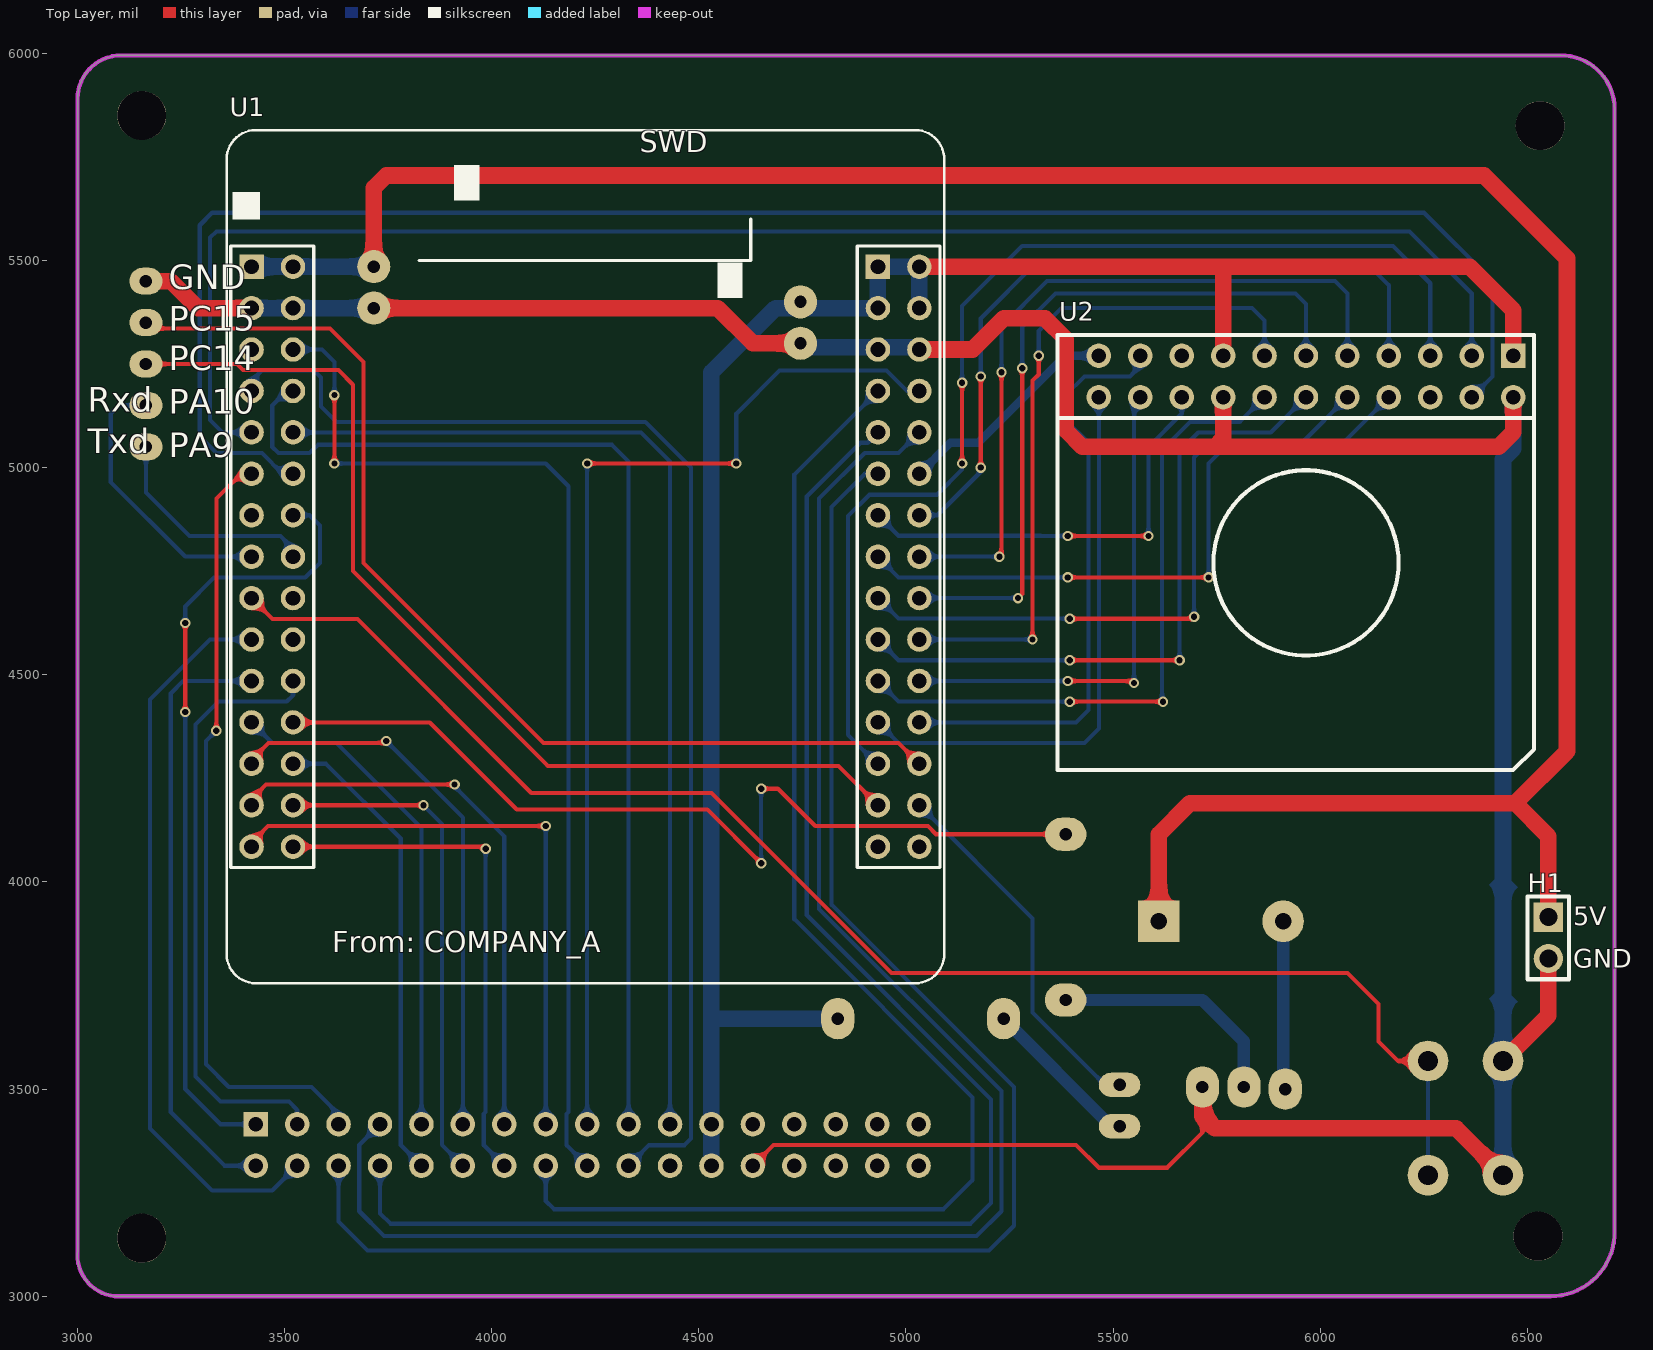
[diagram p0: Top Layer view]
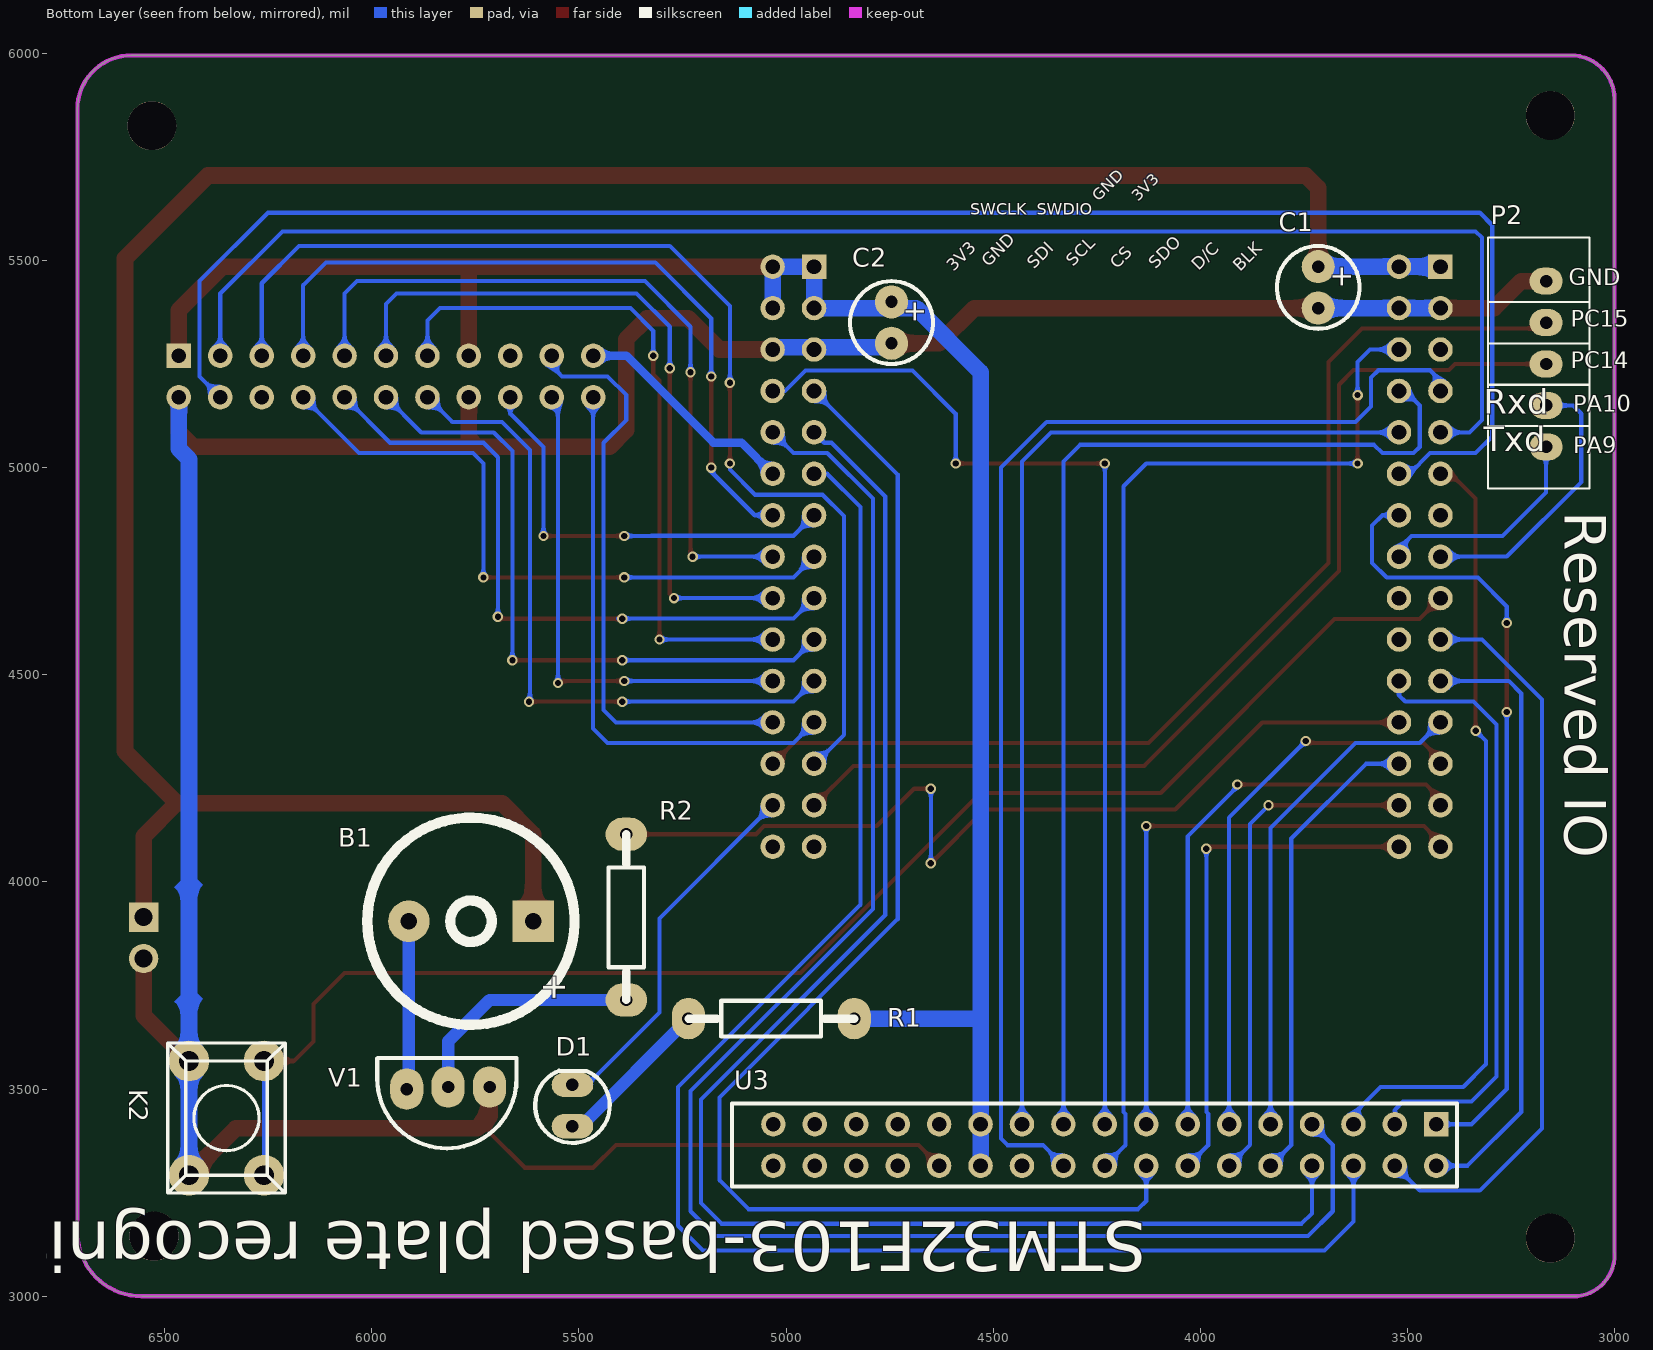
[diagram p1: Bottom Layer view, seen from below]
# Altium PCB MISC89050.pcbdoc
Units mil, origin at the board's own origin, x right, y up, seen from the top; angles counter-clockwise.
Board outline 3710.5 x 2995 mil, 2 copper layers (Top Layer, Bottom Layer); 13 components, 55 nets, 146 pads, 36 vias.

## Layer stack, top to bottom (the 12.6 mil dielectric is the usual default, probably not edited)
Top Solder Mask Layer: solder mask 0.4, Solder Resist, Dk 3.5
Top Layer: signal copper 1.4
Dielectric1: surface 12.6, FR-4, Dk 4.8
Bottom Layer: signal copper 1.4
Bottom Solder Mask Layer: solder mask 0.4, Solder Resist, Dk 3.5

## Board outline
3090.5,3000 6555.5,3000 ccw(c6555.5,3155) 6710.5,3155 6710.5,5865 ccw(c6580.5,5865) 6580.5,5995 3105.5,5995 ccw(c3105.5,5890) 3000.5,5890 3000.5,3110 ccw(c3100.5,3100) 3090.5,3000

## Design rules (kind name [scope] priority, off if disabled: settings)
BoardOutlineClearance Plane_innerPlane_1 [All] p2 off: genericclearance=6 ignorepadtopadclearanceinfootprint=FALSE except(0: Arc-SplitContinuation Track-SplitContinuation SMDPad-SplitContinuation THPad-SplitContinuation Via-SplitContinuation Fill-SplitContinuation Region-SplitContinuation Poly-SplitContinuation Text-SplitContinuation Hole-SplitContinuation; 6: Arc-CutoutEdge Track-CutoutEdge SMDPad-CutoutEdge THPad-CutoutEdge Via-CutoutEdge Fill-CutoutEdge Region-CutoutEdge Text-CutoutEdge; 6.9: Hole-OutlineEdge Hole-CutoutEdge; 10: Poly-OutlineEdge Poly-CutoutEdge; 11.8: Arc-OutlineEdge Track-OutlineEdge SMDPad-OutlineEdge THPad-OutlineEdge Via-OutlineEdge Fill-OutlineEdge Region-OutlineEdge Text-OutlineEdge)
BoardOutlineClearance Copper_copperRegion_1 [All] p4 off: genericclearance=6 ignorepadtopadclearanceinfootprint=FALSE except(0: Arc-SplitContinuation Track-SplitContinuation SMDPad-SplitContinuation THPad-SplitContinuation Via-SplitContinuation Fill-SplitContinuation Region-SplitContinuation Poly-SplitContinuation Text-SplitContinuation Hole-SplitContinuation; 6: Arc-CutoutEdge Track-CutoutEdge SMDPad-CutoutEdge THPad-CutoutEdge Via-CutoutEdge Fill-CutoutEdge Region-CutoutEdge Text-CutoutEdge; 6.9: Hole-OutlineEdge Hole-CutoutEdge; 10: Poly-OutlineEdge Poly-CutoutEdge; 11.8: Arc-OutlineEdge Track-OutlineEdge SMDPad-OutlineEdge THPad-OutlineEdge Via-OutlineEdge Fill-OutlineEdge Region-OutlineEdge Text-OutlineEdge)
BoardOutlineClearance safeClearance_1 [All] p6: genericclearance=6 ignorepadtopadclearanceinfootprint=FALSE except(0: Arc-SplitContinuation Track-SplitContinuation SMDPad-SplitContinuation THPad-SplitContinuation Via-SplitContinuation Fill-SplitContinuation Region-SplitContinuation Poly-SplitContinuation Text-SplitContinuation Hole-SplitContinuation; 6: Arc-CutoutEdge Track-CutoutEdge SMDPad-CutoutEdge THPad-CutoutEdge Via-CutoutEdge Fill-CutoutEdge Region-CutoutEdge Text-CutoutEdge; 6.9: Hole-OutlineEdge Hole-CutoutEdge; 10: Poly-OutlineEdge Poly-CutoutEdge; 11.8: Arc-OutlineEdge Track-OutlineEdge SMDPad-OutlineEdge THPad-OutlineEdge Via-OutlineEdge Fill-OutlineEdge Region-OutlineEdge Text-OutlineEdge)
Clearance Plane_innerPlane [All] p1 off: gap=6 ignorepadtopadclearanceinfootprint=FALSE except(6.9: Hole-Track Hole-SMDPad Hole-THPad Hole-Via Fill-Hole Region-Hole Hole-Arc Hole-Text; 10: Poly-Track Poly-SMDPad Poly-THPad Poly-Via Poly-Fill Poly-Region Poly-Poly Poly-Arc Poly-Text Poly-Hole)
Clearance Copper_copperRegion [All] p3 off: gap=6 ignorepadtopadclearanceinfootprint=FALSE except(6.9: Hole-Track Hole-SMDPad Hole-THPad Hole-Via Fill-Hole Region-Hole Hole-Arc Hole-Text; 10: Poly-Track Poly-SMDPad Poly-THPad Poly-Via Poly-Fill Poly-Region Poly-Poly Poly-Arc Poly-Text Poly-Hole)
Clearance safeClearance [All] p5: gap=6 ignorepadtopadclearanceinfootprint=FALSE except(6.9: Hole-Track Hole-SMDPad Hole-THPad Hole-Via Fill-Hole Region-Hole Hole-Arc Hole-Text; 10: Poly-Track Poly-SMDPad Poly-THPad Poly-Via Poly-Fill Poly-Region Poly-Poly Poly-Arc Poly-Text Poly-Hole)
DiffPairsRouting differentialPair [All] p1: maxlimit=6 minlimit=6 mostfreqgap=6 toplayer_minwidth=5 toplayer_prefwidth=10 toplayer_maxwidth=100 toplayer_mingap=6 toplayer_prefgap=6 toplayer_maxgap=6 bottomlayer_minwidth=5 bottomlayer_prefwidth=10 bottomlayer_maxwidth=100 bottomlayer_mingap=6 bottomlayer_prefgap=6 bottomlayer_maxgap=6 maxuncoupledlength=10
Length netLength [All] p1: minlimit=0 maxlimit=0
PasteMaskExpansion pasteMaskExpansion [All] p1: expansion=0
PlaneConnect innerPlane [All] p1: planeconnectstyle=Relief reliefexpansion=20 reliefentries=4 reliefconductorwidth=10 reliefairgap=10
PolygonConnect copperRegion [All] p1: connectstyle=Relief reliefconductorwidth=10 reliefentries=4 polygonreliefangle="90 Angle" airgapwidth=10 via.connectstyle=Relief via.reliefconductorwidth=10 via.reliefentries=4 via.polygonreliefangle="90 Angle" via.airgapwidth=10
RoutingVias viaSize [All] p1: holewidth=12.01 width=24.02 viastyle="Through Hole" minholewidth=11.81 minwidth=19.68 maxholewidth=236.22 maxwidth=393.7
SolderMaskExpansion solderMaskExpansion [IsVia] p1: expansion=-1000 istentingtop=TRUE
SolderMaskExpansion solderMaskExpansion [All] p2: expansion=2 istentingtop=FALSE
Width trackWidth [All] p1: maxlimit=100 minlimit=5 preferedwidth=10
1 further rules are at their usual default settings.

## Components (designator, comment, footprint, x,y, rotation, side; value= is the part's Value field where it differs from the comment)
B1 "Buzzer FMQ" 蜂鸣器 5610.5,3905 r0 bottom
C1 "10uf" CD0.254cm 3710.5,5435 r270 bottom
C2 "10uf" CD0.254cm 4740.5,5350 r270 bottom
D1 "LED" 发光二极管FZ 5515.5,3410 r90 bottom
H1 "" HDR-TH_2P-P2.54-V-M-1 6550.5,3865 r270 top
K2 "Key button" 按键 6350.5,3430 r270 bottom
P2 "5P" 5ZHEN-100mil 3165.5,5050 r0 bottom
R1 "1K" 电阻FZ 4835.5,3670 r0 bottom
R2 "10K" 电阻FZ 5385.5,4115 r270 bottom
U1 "STM32F103RCT6 core board" "STM32F103RC/RB 核心板" 5055.29,3790 r0 top
U2 "OV7670 with FIFO" OV7670模块 6465.5,5270 r180 top
U3 "TFT_ILI9341 2.8" 2.8寸TFT 3430.5,3415 r0 bottom
V1 "Transistor 3" 三极管FZ 5815.5,3505 r0 bottom

## Footprints (in the part's own frame and the unit in brackets; to place one, negate y for a bottom-side part, rotate by r counter-clockwise, add the part's x,y. Pads: shape width x height; smd on the part's side, far side on the other; paste and mask are expansions set on the pad)
2.8寸TFT [mm]
  rect 1.5x1.5 hole 0.9: 1(0,0)
  round 1.5 hole 0.9: 2(0,2.54) 3(2.54,0) 4(2.54,2.54) 5(5.08,0) 6(5.08,2.54) 7(7.62,0) 8(7.62,2.54) 9(10.16,0) 10(10.16,2.54) 11(12.7,0) 12(12.7,2.54) 13(15.24,0) 14(15.24,2.54) 15(17.78,0) 16(17.78,2.54) 17(20.32,0) 18(20.32,2.54) 19(22.86,0) 20(22.86,2.54) 21(25.4,0) 22(25.4,2.54) 23(27.94,0) 24(27.94,2.54) 25(30.48,0) 26(30.48,2.54) 27(33.02,0) 28(33.02,2.54) 29(35.56,0) 30(35.56,2.54) 31(38.1,0) 32(38.1,2.54) 33(40.64,0) 34(40.64,2.54)
  silkscreen extent -1.27,-1.27 43.18,3.81
5ZHEN-100mil [mil]
  oval 80x65 hole 30: 1(0,0) 2(0,-100) 3(0,-200) 4(0,-300) 5(0,-400)
  silkscreen extent -105,-505 140,100
CD0.254cm [mil]
  round 80 hole 30: 1(-50,-5) 2(50,-5)
  silkscreen extent -100,-105 100,95
HDR-TH_2P-P2.54-V-M-1 [mm]
  rect 1.8x1.8 hole 1.1: 1(-1.27,0)
  round 1.8 hole 1.1: 2(1.27,0)
  silkscreen extent -2.54,-1.27 2.54,1.27
OV7670模块 [mm]
  rect 1.5x1.5 hole 0.9: 1(0,0)
  round 1.5 hole 0.9: 2(0,2.54) 3(2.54,0) 4(2.54,2.54) 5(5.08,0) 6(5.08,2.54) 7(7.62,0) 8(7.62,2.54) 9(10.16,0) 10(10.16,2.54) 11(12.7,0) 12(12.7,2.54) 13(15.24,0) 14(15.24,2.54) 15(17.78,0) 16(17.78,2.54) 17(20.32,0) 18(20.32,2.54) 19(22.86,0) 20(22.86,2.54) 21(25.4,0) 22(25.4,2.54)
  silkscreen extent -1.27,-1.27 27.94,25.4
"STM32F103RC/RB 核心板" [mm]
  rect 1.5x1.5 hole 0.9: 1(-41.524,43.053) 31(-3.122,43.053)
  round 1.5 hole 0.9: 2(-38.984,43.053) 3(-41.524,40.513) 4(-38.984,40.513) 5(-41.524,37.973) 6(-38.984,37.973) 7(-41.524,35.433) 8(-38.984,35.433) 9(-41.524,32.893) 10(-38.984,32.893) 11(-41.524,30.353) 12(-38.984,30.353) 13(-41.524,27.813) 14(-38.984,27.813) 15(-41.524,25.273) 16(-38.984,25.273) 17(-41.524,22.733) 18(-38.984,22.733) 19(-41.524,20.193) 20(-38.984,20.193) 21(-41.524,17.653) 22(-38.984,17.653) 23(-41.524,15.113) 24(-38.984,15.113) 25(-41.524,12.573) 26(-38.984,12.573) 27(-41.524,10.033) 28(-38.984,10.033) 29(-41.524,7.493) 30(-38.984,7.493) 32(-0.582,43.053) 33(-3.122,40.513) 34(-0.582,40.513) 35(-3.122,37.973) 36(-0.582,37.973) 37(-3.122,35.433) 38(-0.582,35.433) 39(-3.122,32.893) 40(-0.582,32.893) 41(-3.122,30.353) 42(-0.582,30.353) 43(-3.122,27.813) 44(-0.582,27.813) 45(-3.122,25.273) 46(-0.582,25.273) 47(-3.122,22.733) 48(-0.582,22.733) 49(-3.122,20.193) 50(-0.582,20.193) 51(-3.122,17.653) 52(-0.582,17.653) 53(-3.122,15.113) 54(-0.582,15.113) 55(-3.122,12.573) 56(-0.582,12.573) 57(-3.122,10.033) 58(-0.582,10.033) 59(-3.122,7.493) 60(-0.582,7.493)
  silkscreen extent -43.05,-0.88 0.95,51.42
三极管FZ [mil]
  oval 80x100 hole 30: 1(0,0) 2(-100,0) 3(100,5)
  silkscreen extent -165,-70 171,148
发光二极管FZ [mil]
  oval 59.06x100 hole 30: 1(0,0) 2(100,0)
  silkscreen extent -40,-90 134,90
按键 [mm]
  round 2.5 hole 1.2: 1(-3.5,2.3) 1(3.5,2.3) 2(-3.5,-2.3) 2(3.5,-2.3)
  silkscreen extent -4.6,-3.6 4.6,3.6
电阻FZ [mil]
  oval 80x100 hole 30: 1(0,0) 2(400,0)
  silkscreen extent 0,-43 400,43
蜂鸣器 [mil]
  rect 100x100 hole 40: 1(0,0)
  round 100 hole 40: 2(300,0)
  silkscreen extent -100,-250 400,250

## Free pads (board coordinates)
  round 118.11 hole 118.11: ""(3155.5,3140) ""(3155.5,5850) ""(6525.5,3145) ""(6530.5,5825)

## Via types
v1: diameter 25, hole 15, Top Layer to Bottom Layer, 36 vias

## Nets (pads, with @x,y where several pads share a name; then routed paths per layer and width w, separated by ;. In a path a pad name is that pad's centre, name@x,y a point inside that pad or via, vN(x,y) a via of type N, cw(c..) or ccw(c..) an arc to the next point about the centre after c; other vN are vias at no path point)
5V: B1.1 C1.1 H1.1 U1.1 U1.2 | length 6236.2
  Top Layer w40: C1.1 3715.5,5675 3745.5,5705 6395.5,5705 6595.5,5505 6595.5,4315 6470.5,4190 ; B1.1 5610.5,4115 5685.5,4190 6470.5,4190 ; H1.1 6550.5,4110 6470.5,4190
  Bottom Layer w40: U1.1 U1.2 C1.1
$1N58: U1.18
$1N59: U1.20 | length 15
  Bottom Layer w10: U1.20 U1.20@3520.5,4600
$1N76: U1.59
$1N88: U1.60
$1N92: B1.2 V1.3 | length 407.1
  Bottom Layer w30: B1.2 5910.5,3505 V1.3
$1N481: D1.1 R1.2 | length 387.7
  Bottom Layer w30: R1.2 5495.5,3410 D1.1
$1N484: R2.2 V1.1 | length 581.4
  Bottom Layer w30: R2.2 5715.5,3715 5815.5,3615 V1.1
GND: C1.2 C2.2 H1.2 K2.2 P2.5 U1.3 U1.4 U1.35 U1.36 U2.2 U2.16 U3.26 V1.2 | length 8119.2
  Top Layer w10: U3.26 4680.5,3365 5410.5,3365 5465.5,3310 5630.5,3310 5715.5,3395 5715.5,3435
  Top Layer w40: P2.5 3225.5,5450 3290.5,5385 U1.3 ; C1.2 4545.5,5385 4630.5,5300 C2.2 ; U1.36 5160.5,5285 5235.5,5360 5335.5,5360 5385.5,5310 5385.5,5090 5425.5,5050 5745.5,5050 ; V1.2 5715.5,3435 5745.5,3405 6328.25,3405 K2.2@6441.05,3292.2 ; U2.16 5765.5,5070 5745.5,5050 ; K2.2@6441.05,3567.8 6550.5,3677.24 H1.2 ; U2.2 6465.5,5085 6430.5,5050 5745.5,5050
  Bottom Layer w40: U1.3 U1.4 C1.2 ; C2.2@4745.5,5290 5027.37,5290 U1.36 ; K2.2@6441.05,3292.2 6441.05,3567.8 6441.05,5020.55 6465.5,5045 U2.2
PA0: U1.51 U2.14 | length 1617.7
  Top Layer w10: v1(5395.5,4435) v1(5620.5,4435)
  Bottom Layer w10: U1.51 4982.37,4435 v1(5395.5,4435) ; v1(5620.5,4435) 5618,4437.5 5618,5042.5 5685.5,5110 5805.5,5110 U2.14
PA1: U1.50 U2.13 | length 1689.6
  Top Layer w10: v1(5305.5,4585) 5305.5,5210 5320.5,5225 v1(5320.5,5270)
  Bottom Layer w10: U1.50 v1(5305.5,4585) ; v1(5320.5,5270) 5320.5,5330 5375.5,5385 5835.5,5385 5865.5,5355 U2.13
PA2: U1.49 U2.12 | length 1612.7
  Top Layer w10: v1(5395.5,4535) v1(5660.5,4535)
  Bottom Layer w10: U1.49 4982.37,4535 v1(5395.5,4535) ; v1(5660.5,4535) 5660.5,5040 5705.5,5085 5880.5,5085 U2.12
PA3: U1.48 U2.11 | length 1750.8
  Top Layer w10: v1(5270.5,4685) 5280.5,4695 v1(5280.5,5240)
  Bottom Layer w10: U1.48 v1(5270.5,4685) ; v1(5280.5,5240) 5280.5,5340 5360.5,5420 5940.5,5420 5965.5,5395 U2.11
PA4: U1.47 U2.10 | length 1627.1
  Top Layer w10: v1(5395.5,4635) 5690.5,4635 v1(5695.5,4640)
  Bottom Layer w10: U1.47 4981.89,4635.47 5405.03,4635.47 5404.55,4635 v1(5395.5,4635) ; v1@5700.5,4635 v1(5695.5,4640) 5695.5,5025 5730.5,5060 5955.5,5060 U2.10
PA5: U1.46 U2.9 | length 1800.3
  Top Layer w10: v1(5225.5,4785) 5230.5,4790 v1(5230.5,5230)
  Bottom Layer w10: U1.46 v1(5225.5,4785) v1@5230.5,4790 ; v1(5230.5,5230) 5230.5,5340 5340.5,5450 6035.5,5450 6065.5,5420 U2.9
PA6: U1.45 U2.8 | length 1595.1
  Top Layer w10: v1(5390.5,4735) v1(5730.5,4735)
  Bottom Layer w10: U1.45 4982.37,4735 v1(5390.5,4735) ; v1(5730.5,4735) 5730.5,5010 5755.5,5035 6030.5,5035 U2.8
PA7: U1.44 U2.7 | length 1795.3
  Top Layer w10: v1(5180.5,5000) v1(5180.5,5220)
  Bottom Layer w10: U1.44 5075.5,4885 5180.5,4990 v1(5180.5,5000) ; v1(5180.5,5220) 5180.5,5360 5315.5,5495 6110.5,5495 6165.5,5440 U2.7
PA8: U1.13
PA9: P2.1 U1.16 | length 540.9
  Bottom Layer w10: P2.1 3165.5,4940 3270.5,4835 3490.5,4835 3520.5,4805 U1.16
PA10: P2.2 U1.15 | length 672.8
  Bottom Layer w10: P2.2 3100.5,5150 3080.5,5130 3080.5,4965 3260.5,4785 U1.15
PA12: K2.1 U1.17 | length 3630.5
  Top Layer w10: U1.17 3470.97,4634.53 3675.97,4634.53 4095.5,4215 4530.5,4215 4965.5,3780 6065.5,3780 6140.5,3705 6140.5,3615 6187.7,3567.8 K2.1@6259.95,3567.8
  Bottom Layer w10: K2.1@6259.95,3292.2 K2.1@6259.95,3567.8
PB0: U1.41 U3.6 | length 3881.1
  Bottom Layer w10: U3.6 3630.5,3180 3700.5,3110 5200.5,3110 5260.5,3170 5260.5,3505 4820.5,3945 4820.5,4905 4900.5,4985 U1.41
PB1: U1.40 U3.7 | length 4040.8
  Bottom Layer w10: U3.7 3680.5,3365 3680.5,3205 3740.5,3145 5170.5,3145 5230.5,3205 5230.5,3495 4790.5,3935 4790.5,4925 4900.5,5035 4982.37,5035 U1.40
PB2: U1.39 U3.8 | length 3746.7
  Bottom Layer w10: U3.8 3730.5,3200 3755.5,3175 5155.5,3175 5205.5,3225 5205.5,3475 4760.5,3920 4760.5,4930.36 4890.14,5060 4907.37,5060 U1.39
PB3: U1.23 U3.9 | length 1230.6
  Bottom Layer w10: U1.23 3470.5,4335 3625.5,4335 3830.5,4130 U3.9
PB4: U1.26 U3.10 | length 1145.3
  Bottom Layer w10: U1.26 3600.5,4285 3780.5,4105 3780.5,3365 U3.10
PB5: U1.25 U3.11 | length 1362.3
  Top Layer w10: U1.25 3420.5,4295 3460.97,4335.47 3740.97,4335.47 v1(3745.5,4340)
  Bottom Layer w10: v1@3740.5,4345 v1(3745.5,4340) 3930.5,4155 U3.11
PB6: U1.28 U3.12 | length 1210.1
  Top Layer w10: U1.28 v1(3835.5,4185)
  Bottom Layer w10: 3845.32,4174.82 3880.03,4140.12 3880.03,3365.47 U3.12
PB7: U1.27 U3.13 | length 1389.2
  Top Layer w10: U1.27 3420.5,4200 3455.5,4235 v1(3910.5,4235)
  Bottom Layer w10: v1(3910.5,4235) 3910.5,4230 4030.5,4110 U3.13
PB8: U1.30 U3.14 | length 1261.5
  Top Layer w10: U1.30 3980.5,4085 v1(3985.5,4080)
  Bottom Layer w10: v1@3980.5,4075 v1(3985.5,4080) 3985.5,3444.57 3980.97,3440.04 3980.97,3364.53 U3.14
PB9: U1.29 U3.15 | length 1456.6
  Top Layer w10: U1.29 3420.5,4095 3460.5,4135 v1(4130.5,4135)
  Bottom Layer w10: U3.15 v1(4130.5,4135)
PB10: U1.37 U3.16 | length 3319
  Bottom Layer w10: U3.16 4130.5,3230 4150.5,3210 5090.5,3210 5160.5,3280 5160.5,3480 4730.5,3910 4730.5,4983.13 U1.37
PB11: U1.38 U3.17 | length 2580.7
  Top Layer w10: v1(4230.5,5010) v1(4590.5,5010)
  Bottom Layer w10: U3.17 v1(4230.5,5010) ; v1(4590.5,5010) 4590.5,5130 4695.03,5234.53 4952.88,5234.53 5002.41,5185 U1.38
PB12: U1.6 U3.18 | length 2607.6
  Top Layer w10: v1(3620.5,5010) v1(3620.5,5175)
  Bottom Layer w10: U1.6 3590.5,5285 3620.5,5255 v1(3620.5,5175) ; v1(3620.5,5010) 4130.5,5010 4185.5,4955 4185.5,3444.57 4180.97,3440.04 4180.97,3364.53 U3.18
PB13: U1.8 U3.19 | length 2655.6
  Bottom Layer w10: U1.8 3505.5,5185 3470.5,5150 3470.5,5050 3485.5,5035 3560.5,5035 3580.5,5055 4290.5,5055 4330.5,5015 U3.19
PB14: U1.7 U3.20 | length 3031.2
  Bottom Layer w10: U1.7 3420.5,5210 3445.5,5235 3570.5,5235 3588,5217.5 3588,5147.5 3625.5,5110 4370.85,5110 4480.97,4999.88 4480.97,3380.47 4465.03,3364.53 4380.03,3364.53 U3.20
PB15: U1.10 U3.21 | length 2539
  Bottom Layer w10: U1.10 4360.5,5085 4430.5,5015 U3.21
PC0: U1.55 U2.5 | length 2747.7
  Top Layer w10: v1(5135.5,5010) v1(5135.5,5205)
  Bottom Layer w10: U1.55 4930.5,4285 4860.5,4355 4860.5,4883.18 4911.85,4934.53 5075.03,4934.53 5135.5,4995 v1(5135.5,5010) ; v1(5135.5,5205) 5135.5,5390 5280.5,5535 6175.5,5535 6265.5,5445 U2.5
PC1: U1.54 U2.19 | length 1437.3
  Bottom Layer w10: U1.54 5410.5,4385 5440.5,4415 5440.5,5060 5385.5,5115 5385.5,5175 5430.5,5220 5540.5,5220 5565.5,5245 U2.19
PC2: U1.53 U2.22 | length 1368.3
  Bottom Layer w10: U1.53 4982.37,4335 5430.5,4335 5465.5,4370 U2.22
PC3: U1.52 U2.20 | length 1210.2
  Top Layer w10: v1(5390.5,4485) 5545.5,4485 v1(5550.5,4480)
  Bottom Layer w10: U1.52 v1(5390.5,4485) ; v1(5550.5,4480) U2.20@5550.5,5170
PC4: U1.43 U2.18 | length 1042
  Top Layer w10: v1(5390.5,4835) v1(5585.5,4835)
  Bottom Layer w10: U1.43 4981.89,4835.47 5325.03,4835.47 5325.5,4835 v1(5390.5,4835) ; v1(5585.5,4835) 5585.5,5050 5665.5,5130 U2.18
PC5: U1.42 U2.21 | length 551.2
  Bottom Layer w20: U1.42 5107.37,5060 5175.5,5060 5385.5,5270 U2.21
PC6: U1.9 U2.3 | length 3815.8
  Bottom Layer w10: U1.9 3350.5,5085 3320.5,5115 3320.5,5555 3335.5,5570 6215.5,5570 6365.5,5420 U2.3
PC7: U1.12 U2.4 | length 4273.8
  Bottom Layer w10: U1.12 3495.5,4985 3445.5,5035 3335.5,5035 3295.5,5075 3295.5,5585 3325.5,5615 6250.5,5615 6415.5,5450 6415.5,5220 U2.4
PC8: U1.11 U3.5 | length 1879.9
  Top Layer w10: v1(3335.5,4365) 3335.5,4925 3395.5,4985 U1.11
  Bottom Layer w10: v1(3335.5,4365) 3310.5,4340 3310.5,3560 3365.5,3505 3565.5,3505 3630.5,3440 U3.5
PC9: U1.14 U3.1 | length 1904.1
  Top Layer w10: v1(3260.5,4410) v1(3260.5,4625)
  Bottom Layer w10: v1(3260.5,4410) 3260.5,3500 3345.5,3415 U3.1 ; v1(3260.5,4625) 3260.5,4665 3330.03,4734.53 3550.03,4734.53 3585.5,4770 3585.5,4860 3560.5,4885 U1.14
PC10: U1.19 U3.4 | length 1782.3
  Bottom Layer w10: U1.19 3320.14,4585 3175.5,4440.36 3175.5,3405 3325.5,3255 3470.5,3255 U3.4
PC11: U1.22 U3.3 | length 1462.1
  Bottom Layer w10: U1.22 3520.5,4450 3505.5,4435 3340.5,4435 3285.5,4380 3285.5,3530 3345.5,3470 3510.5,3470 3530.5,3450 U3.3
PC12: U1.21 U3.2 | length 1476.3
  Bottom Layer w10: U1.21 3255.5,4485 3225.5,4455 3225.5,3445 3355.5,3315 U3.2
PC13: D1.2 U1.58 | length 895.6
  Bottom Layer w10: U1.58 5305.5,3911.87 5305.5,3685 5480.5,3510 D1.2
PC14: P2.3 U1.57 | length 2471.6
  Top Layer w10: P2.3 3385.46,5250 3399.98,5235.47 3630.03,5235.47 3665.5,5200 3665.5,4750 4135.5,4280 4837.37,4280 U1.57
PC15: P2.4 U1.56 | length 2592.1
  Top Layer w10: P2.4 3180.03,5335.47 3610.03,5335.47 3690.5,5255 3690.5,4770 4125.03,4335.47 4981.89,4335.47 U1.56
PD2: R2.1 U1.24 | length 2231.4
  Top Layer w10: U1.24 3850.5,4385 4060.5,4175 4520.5,4175 v1(4650.5,4045) ; v1(4650.5,4225) 4690.5,4225 4780.97,4134.53 5052.88,4134.53 5072.41,4115 R2.1
  Bottom Layer w10: v1(4650.5,4045) v1(4650.5,4225)
VCC_3.3V: C2.1 R1.1 U1.31 U1.32 U1.33 U1.34 U2.1 U2.15 U3.23 U3.24 | length 4789.8
  Top Layer w40: U1.32 5765.5,5485 ; U2.15 5765.5,5485 ; U2.1 6465.5,5380 6360.5,5485 5765.5,5485
  Bottom Layer w40: U3.24 U3.23 4530.5,3675 ; R1.1 4535.5,3670 4530.5,3675 ; U1.34 U1.32 U1.31 U1.33 4685.5,5385 4530.5,5230 4530.5,3675
pads on no net: U1.5 U2.6 U2.17 U3.22 U3.25 U3.27 U3.28 U3.29 U3.30 U3.31 U3.32 U3.33 U3.34

## Keep-outs
Board Outline Layer:
  the board outline again, w10

## Other copper
Top Layer:
  region net GND: 5715.5,3435 5720.5,3395 5720.61,3396.17 5720.93,3396.98 5721.48,3397.45 5722.24,3397.56 5723.21,3397.32 5724.41,3396.73 5725.82,3395.79 5727.45,3394.5 5729.29,3392.85 5731.36,3390.86 5759.64,3419.14 5755.05,3424.13 5750.95,3429.43 5747.33,3435.05 5744.19,3440.99 5741.53,3447.25 5739.36,3453.82 5737.67,3460.71 5736.46,3467.92 5735.74,3475.44 5735.5,3483.28
  region net GND: 5710.5,3395 5710.39,3397.75 5710.06,3400.5 5709.52,3403.26 5708.76,3406.03 5707.79,3408.8 5706.59,3411.59 5705.18,3414.38 5703.56,3417.18 5701.71,3419.99 5699.65,3422.8 5731.35,3422.8 5729.29,3419.99 5725.81,3414.38 5724.4,3411.59 5723.21,3408.8 5722.23,3406.03 5721.48,3403.26 5720.93,3400.5 5720.61,3397.75 5720.5,3395
  region net GND: 5710.5,3395 5710.39,3397.75 5710.06,3400.5 5709.52,3403.26 5708.76,3406.03 5707.79,3408.8 5706.59,3411.59 5705.18,3414.38 5703.56,3417.18 5701.71,3419.99 5699.65,3422.8 5731.35,3422.8 5729.29,3419.99 5725.81,3414.38 5724.4,3411.59 5723.21,3408.8 5722.23,3406.03 5721.48,3403.26 5720.93,3400.5 5720.61,3397.75 5720.5,3395
  region net PD2: 4640.63,4061.94 4641.54,4061.09 4642.46,4060.32 4643.39,4059.65 4644.35,4059.07 4645.31,4058.58 4646.29,4058.18 4647.29,4057.88 4648.3,4057.66 4649.33,4057.53 4650.37,4057.5 4638,4045.12 4637.96,4046.17 4637.84,4047.2 4637.62,4048.21 4637.31,4049.2 4636.92,4050.19 4636.43,4051.15 4635.85,4052.1 4635.17,4053.04 4634.41,4053.96 4633.56,4054.87
  region net PD2: 4669.46,4220 4668.21,4219.96 4667.02,4219.85 4665.88,4219.66 4664.8,4219.4 4663.77,4219.06 4662.79,4218.65 4661.87,4218.16 4661,4217.6 4660.19,4216.96 4659.43,4216.25 4659.43,4233.75 4660.19,4233.04 4661,4232.4 4661.87,4231.84 4662.79,4231.35 4663.77,4230.94 4664.8,4230.6 4665.88,4230.34 4667.02,4230.15 4668.21,4230.04 4669.46,4230
  region net PB12: 3625.5,5028.96 3625.54,5027.71 3625.65,5026.52 3625.84,5025.39 3626.1,5024.3 3626.44,5023.27 3626.85,5022.3 3627.34,5021.37 3627.9,5020.5 3628.54,5019.69 3629.25,5018.93 3611.75,5018.93 3612.46,5019.69 3613.1,5020.5 3613.66,5021.37 3614.15,5022.3 3614.56,5023.27 3614.9,5024.3 3615.16,5025.39 3615.35,5026.52 3615.46,5027.71 3615.5,5028.96
  region net PB12: 3615.5,5156.04 3615.46,5157.29 3615.35,5158.48 3615.16,5159.61 3614.9,5160.7 3614.56,5161.73 3614.15,5162.7 3613.66,5163.63 3613.1,5164.5 3612.46,5165.31 3611.75,5166.07 3629.25,5166.07 3628.54,5165.31 3627.9,5164.5 3627.34,5163.63 3626.85,5162.7 3626.44,5161.73 3626.1,5160.7 3625.84,5159.61 3625.65,5158.48 3625.54,5157.29 3625.5,5156.04
  region net PB11: 4571.54,5015 4572.79,5015.04 4573.98,5015.15 4575.11,5015.34 4576.2,5015.6 4577.23,5015.94 4578.2,5016.35 4579.13,5016.84 4579.99,5017.4 4580.81,5018.04 4581.57,5018.75 4581.57,5001.25 4580.81,5001.96 4579.99,5002.6 4579.13,5003.16 4578.2,5003.65 4577.23,5004.06 4576.2,5004.4 4575.11,5004.66 4573.98,5004.85 4572.79,5004.96 4571.54,5005
  region net PB11: 4249.46,5005 4248.21,5004.96 4247.02,5004.85 4245.88,5004.66 4244.8,5004.4 4243.77,5004.06 4242.79,5003.65 4241.87,5003.16 4241,5002.6 4240.19,5001.96 4239.43,5001.25 4239.43,5018.75 4240.19,5018.04 4241,5017.4 4241.87,5016.84 4242.79,5016.35 4243.77,5015.94 4244.8,5015.6 4245.88,5015.34 4247.02,5015.15 4248.21,5015.04 4249.46,5015
  region net PA0: 5601.54,4440 5602.79,4440.04 5603.98,4440.15 5605.11,4440.34 5606.2,4440.6 5607.23,4440.94 5608.2,4441.35 5609.13,4441.84 5609.99,4442.4 5610.81,4443.04 5611.57,4443.75 5611.57,4426.25 5610.81,4426.96 5609.99,4427.6 5609.13,4428.16 5608.2,4428.65 5607.23,4429.06 5606.2,4429.4 5605.11,4429.66 5603.98,4429.85 5602.79,4429.96 5601.54,4430
  region net PA5: 5235.5,4800 5235.51,4798.74 5235.75,4795.27 5235.89,4794.22 5236.27,4792.27 5236.51,4791.37 5237.07,4789.72 5221.05,4796.68 5221.9,4797.07 5222.65,4797.56 5223.32,4798.14 5223.9,4798.83 5224.39,4799.61 5224.79,4800.49 5225.1,4801.47 5225.32,4802.55 5225.45,4803.72 5225.5,4805
  region net PA7: 5185.5,5018.96 5185.54,5017.71 5185.65,5016.52 5185.84,5015.39 5186.1,5014.3 5186.44,5013.27 5186.85,5012.3 5187.34,5011.37 5187.9,5010.5 5188.54,5009.69 5189.25,5008.93 5171.75,5008.93 5172.46,5009.69 5173.1,5010.5 5173.66,5011.37 5174.15,5012.3 5174.56,5013.27 5174.9,5014.3 5175.16,5015.39 5175.35,5016.52 5175.46,5017.71 5175.5,5018.96
  region net PC0: 5140.5,5028.96 5140.54,5027.71 5140.65,5026.52 5140.84,5025.39 5141.1,5024.3 5141.44,5023.27 5141.85,5022.3 5142.34,5021.37 5142.9,5020.5 5143.54,5019.69 5144.25,5018.93 5126.75,5018.93 5127.46,5019.69 5128.1,5020.5 5128.66,5021.37 5129.15,5022.3 5129.56,5023.27 5129.9,5024.3 5130.16,5025.39 5130.35,5026.52 5130.46,5027.71 5130.5,5028.96
  region net PA3: 5275.5,5221.04 5275.46,5222.29 5275.35,5223.48 5275.16,5224.61 5274.9,5225.7 5274.56,5226.73 5274.15,5227.7 5273.66,5228.63 5273.1,5229.5 5272.46,5230.31 5271.75,5231.07 5289.25,5231.07 5288.54,5230.31 5287.9,5229.5 5287.34,5228.63 5286.85,5227.7 5286.44,5226.73 5286.1,5225.7 5285.84,5224.61 5285.65,5223.48 5285.54,5222.29 5285.5,5221.04
  region net PA1: 5315.5,5251.04 5315.46,5252.29 5315.35,5253.48 5315.16,5254.61 5314.9,5255.7 5314.56,5256.73 5314.15,5257.7 5313.66,5258.63 5313.1,5259.5 5312.46,5260.31 5311.75,5261.07 5329.25,5261.07 5328.54,5260.31 5327.9,5259.5 5327.34,5258.63 5326.85,5257.7 5326.44,5256.73 5326.1,5255.7 5325.84,5254.61 5325.65,5253.48 5325.54,5252.29 5325.5,5251.04
  region net PA5: 5225.5,5211.04 5225.46,5212.29 5225.35,5213.48 5225.16,5214.61 5224.9,5215.7 5224.56,5216.73 5224.15,5217.7 5223.66,5218.63 5223.1,5219.5 5222.46,5220.31 5221.75,5221.07 5239.25,5221.07 5238.54,5220.31 5237.9,5219.5 5237.34,5218.63 5236.85,5217.7 5236.44,5216.73 5236.1,5215.7 5235.84,5214.61 5235.65,5213.48 5235.54,5212.29 5235.5,5211.04
  region net PA7: 5175.5,5201.04 5175.46,5202.29 5175.35,5203.48 5175.16,5204.61 5174.9,5205.7 5174.56,5206.73 5174.15,5207.7 5173.66,5208.63 5173.1,5209.5 5172.46,5210.31 5171.75,5211.07 5189.25,5211.07 5188.54,5210.31 5187.9,5209.5 5187.34,5208.63 5186.85,5207.7 5186.44,5206.73 5186.1,5205.7 5185.84,5204.61 5185.65,5203.48 5185.54,5202.29 5185.5,5201.04
  region net PC0: 5130.5,5186.04 5130.46,5187.29 5130.35,5188.48 5130.16,5189.61 5129.9,5190.7 5129.56,5191.73 5129.15,5192.7 5128.66,5193.63 5128.1,5194.5 5127.46,5195.31 5126.75,5196.07 5144.25,5196.07 5143.54,5195.31 5142.9,5194.5 5142.34,5193.63 5141.85,5192.7 5141.44,5191.73 5141.1,5190.7 5140.84,5189.61 5140.65,5188.48 5140.54,5187.29 5140.5,5186.04
  region net PA1: 5310.5,4603.96 5310.54,4602.71 5310.65,4601.52 5310.84,4600.39 5311.1,4599.3 5311.44,4598.27 5311.85,4597.3 5312.34,4596.37 5312.9,4595.5 5313.54,4594.69 5314.25,4593.93 5296.75,4593.93 5297.46,4594.69 5298.1,4595.5 5298.66,4596.37 5299.15,4597.3 5299.56,4598.27 5299.9,4599.3 5300.16,4600.39 5300.35,4601.52 5300.46,4602.71 5300.5,4603.96
  region net PC4: 5566.54,4840 5567.79,4840.04 5568.98,4840.15 5570.11,4840.34 5571.2,4840.6 5572.23,4840.94 5573.2,4841.35 5574.13,4841.84 5574.99,4842.4 5575.81,4843.04 5576.57,4843.75 5576.57,4826.25 5575.81,4826.96 5574.99,4827.6 5574.13,4828.16 5573.2,4828.65 5572.23,4829.06 5571.2,4829.4 5570.11,4829.66 5568.98,4829.85 5567.79,4829.96 5566.54,4830
  region net PA0: 5414.46,4430 5413.21,4429.96 5412.02,4429.85 5410.88,4429.66 5409.8,4429.4 5408.77,4429.06 5407.79,4428.65 5406.87,4428.16 5406,4427.6 5405.19,4426.96 5404.43,4426.25 5404.43,4443.75 5405.19,4443.04 5406,4442.4 5406.87,4441.84 5407.79,4441.35 5408.77,4440.94 5409.8,4440.6 5410.88,4440.34 5412.02,4440.15 5413.21,4440.04 5414.46,4440
  region net PC3: 5409.46,4480 5408.21,4479.96 5407.02,4479.85 5405.88,4479.66 5404.8,4479.4 5403.77,4479.06 5402.79,4478.65 5401.87,4478.16 5401,4477.6 5400.19,4476.96 5399.43,4476.25 5399.43,4493.75 5400.19,4493.04 5401,4492.4 5401.87,4491.84 5402.79,4491.35 5403.77,4490.94 5404.8,4490.6 5405.88,4490.34 5407.02,4490.15 5408.21,4490.04 5409.46,4490
  region net PA2: 5414.46,4530 5413.21,4529.96 5412.02,4529.85 5410.88,4529.66 5409.8,4529.4 5408.77,4529.06 5407.79,4528.65 5406.87,4528.16 5406,4527.6 5405.19,4526.96 5404.43,4526.25 5404.43,4543.75 5405.19,4543.04 5406,4542.4 5406.87,4541.84 5407.79,4541.35 5408.77,4540.94 5409.8,4540.6 5410.88,4540.34 5412.02,4540.15 5413.21,4540.04 5414.46,4540
  region net PA4: 5414.46,4630 5413.21,4629.96 5412.02,4629.85 5410.88,4629.66 5409.8,4629.4 5408.77,4629.06 5407.79,4628.65 5406.87,4628.16 5406,4627.6 5405.19,4626.96 5404.43,4626.25 5404.43,4643.75 5405.19,4643.04 5406,4642.4 5406.87,4641.84 5407.79,4641.35 5408.77,4640.94 5409.8,4640.6 5410.88,4640.34 5412.02,4640.15 5413.21,4640.04 5414.46,4640
  region net PA6: 5409.46,4730 5408.21,4729.96 5407.02,4729.85 5405.88,4729.66 5404.8,4729.4 5403.77,4729.06 5402.79,4728.65 5401.87,4728.16 5401,4727.6 5400.19,4726.96 5399.43,4726.25 5399.43,4743.75 5400.19,4743.04 5401,4742.4 5401.87,4741.84 5402.79,4741.35 5403.77,4740.94 5404.8,4740.6 5405.88,4740.34 5407.02,4740.15 5408.21,4740.04 5409.46,4740
  region net PC4: 5409.46,4830 5408.21,4829.96 5407.02,4829.85 5405.88,4829.66 5404.8,4829.4 5403.77,4829.06 5402.79,4828.65 5401.87,4828.16 5401,4827.6 5400.19,4826.96 5399.43,4826.25 5399.43,4843.75 5400.19,4843.04 5401,4842.4 5401.87,4841.84 5402.79,4841.35 5403.77,4840.94 5404.8,4840.6 5405.88,4840.34 5407.02,4840.15 5408.21,4840.04 5409.46,4840
  region net PA2: 5641.54,4540 5642.79,4540.04 5643.98,4540.15 5645.11,4540.34 5646.2,4540.6 5647.23,4540.94 5648.2,4541.35 5649.13,4541.84 5649.99,4542.4 5650.81,4543.04 5651.57,4543.75 5651.57,4526.25 5650.81,4526.96 5649.99,4527.6 5649.13,4528.16 5648.2,4528.65 5647.23,4529.06 5646.2,4529.4 5645.11,4529.66 5643.98,4529.85 5642.79,4529.96 5641.54,4530
  region net PC3: 5535.5,4490 5536.76,4490.02 5540.22,4490.25 5541.28,4490.39 5543.23,4490.77 5544.13,4491.01 5545.78,4491.58 5538.82,4475.55 5538.43,4476.4 5537.94,4477.15 5537.36,4477.82 5536.67,4478.4 5535.89,4478.89 5535.01,4479.29 5534.03,4479.6 5532.95,4479.82 5531.77,4479.96 5530.5,4480
  region net PA6: 5711.54,4740 5712.79,4740.04 5713.98,4740.15 5715.11,4740.34 5716.2,4740.6 5717.23,4740.94 5718.2,4741.35 5719.13,4741.84 5719.99,4742.4 5720.81,4743.04 5721.57,4743.75 5721.57,4726.25 5720.81,4726.96 5719.99,4727.6 5719.13,4728.16 5718.2,4728.65 5717.23,4729.06 5716.2,4729.4 5715.11,4729.66 5713.98,4729.85 5712.79,4729.96 5711.54,4730
  region net PA4: 5675.5,4640 5676.77,4640.04 5677.95,4640.18 5679.03,4640.4 5680.01,4640.71 5680.89,4641.11 5681.67,4641.6 5682.36,4642.18 5682.94,4642.85 5683.43,4643.6 5683.82,4644.45 5690.78,4628.42 5689.98,4628.72 5689.13,4628.99 5687.28,4629.43 5686.28,4629.61 5684.12,4629.86 5681.76,4629.98 5680.5,4630
  region net PC8: 3340.5,4383.96 3340.54,4382.71 3340.65,4381.52 3340.84,4380.39 3341.1,4379.3 3341.44,4378.27 3341.85,4377.3 3342.34,4376.37 3342.9,4375.5 3343.54,4374.69 3344.25,4373.93 3326.75,4373.93 3327.46,4374.69 3328.1,4375.5 3328.66,4376.37 3329.15,4377.3 3329.56,4378.27 3329.9,4379.3 3330.16,4380.39 3330.35,4381.52 3330.46,4382.71 3330.5,4383.96
  region net PC9: 3265.5,4428.96 3265.54,4427.71 3265.65,4426.52 3265.84,4425.39 3266.1,4424.3 3266.44,4423.27 3266.85,4422.3 3267.34,4421.37 3267.9,4420.5 3268.54,4419.69 3269.25,4418.93 3251.75,4418.93 3252.46,4419.69 3253.1,4420.5 3253.66,4421.37 3254.15,4422.3 3254.56,4423.27 3254.9,4424.3 3255.16,4425.39 3255.35,4426.52 3255.46,4427.71 3255.5,4428.96
  region net PC9: 3255.5,4606.04 3255.46,4607.29 3255.35,4608.48 3255.16,4609.61 3254.9,4610.7 3254.56,4611.73 3254.15,4612.7 3253.66,4613.63 3253.1,4614.5 3252.46,4615.31 3251.75,4616.07 3269.25,4616.07 3268.54,4615.31 3267.9,4614.5 3267.34,4613.63 3266.85,4612.7 3266.44,4611.73 3266.1,4610.7 3265.84,4609.61 3265.65,4608.48 3265.54,4607.29 3265.5,4606.04
  region net PB5: 3725.51,4340.47 3726.78,4340.52 3727.96,4340.65 3729.04,4340.87 3730.03,4341.18 3730.93,4341.58 3731.73,4342.07 3732.44,4342.65 3733.06,4343.32 3733.58,4344.08 3734.01,4344.92 3740.35,4328.61 3739.5,4328.96 3738.61,4329.28 3736.7,4329.8 3735.68,4330.01 3733.5,4330.3 3732.35,4330.4 3729.91,4330.47
  region net PB7: 3891.54,4240 3892.79,4240.04 3893.98,4240.15 3895.11,4240.34 3896.2,4240.6 3897.23,4240.94 3898.2,4241.35 3899.13,4241.84 3899.99,4242.4 3900.81,4243.04 3901.57,4243.75 3901.57,4226.25 3900.81,4226.96 3899.99,4227.6 3899.13,4228.16 3898.2,4228.65 3897.23,4229.06 3896.2,4229.4 3895.11,4229.66 3893.98,4229.85 3892.79,4229.96 3891.54,4230
  region net PB6: 3816.54,4190 3817.79,4190.04 3818.98,4190.15 3820.11,4190.34 3821.2,4190.6 3822.23,4190.94 3823.2,4191.35 3824.13,4191.84 3824.99,4192.4 3825.81,4193.04 3826.57,4193.75 3826.57,4176.25 3825.81,4176.96 3824.99,4177.6 3824.13,4178.16 3823.2,4178.65 3822.23,4179.06 3821.2,4179.4 3820.11,4179.66 3818.98,4179.85 3817.79,4179.96 3816.54,4180
  region net PB9: 4111.54,4140 4112.79,4140.04 4113.98,4140.15 4115.11,4140.34 4116.2,4140.6 4117.23,4140.94 4118.2,4141.35 4119.13,4141.84 4119.99,4142.4 4120.81,4143.04 4121.57,4143.75 4121.57,4126.25 4120.81,4126.96 4119.99,4127.6 4119.13,4128.16 4118.2,4128.65 4117.23,4129.06 4116.2,4129.4 4115.11,4129.66 4113.98,4129.85 4112.79,4129.96 4111.54,4130
  region net PB8: 3970.5,4090 3971.76,4090.02 3975.22,4090.25 3976.28,4090.39 3978.23,4090.77 3979.13,4091.01 3980.78,4091.58 3973.82,4075.55 3973.43,4076.4 3972.94,4077.15 3972.36,4077.82 3971.67,4078.4 3970.89,4078.89 3970.01,4079.29 3969.03,4079.6 3967.95,4079.82 3966.77,4079.96 3965.5,4080
  region net GND: 6402.52,3359.02 6406.1,3355.64 6409.74,3352.62 6413.42,3349.96 6417.15,3347.66 6420.93,3345.72 6424.76,3344.13 6428.64,3342.91 6432.56,3342.05 6436.54,3341.55 6440.56,3341.41 6391.84,3292.7 6391.7,3296.72 6391.2,3300.69 6390.34,3304.62 6389.12,3308.49 6387.54,3312.32 6385.6,3316.1 6383.3,3319.83 6380.64,3323.52 6377.62,3327.15 6374.23,3330.74
  region net PA12: 6187.7,3572.8 6191.03,3573.01 6194.31,3573.67 6197.53,3574.76 6200.71,3576.29 6203.84,3578.26 6206.91,3580.67 6209.94,3583.51 6212.92,3586.79 6215.84,3590.51 6218.72,3594.66 6218.72,3540.93 6215.84,3545.08 6212.92,3548.8 6209.94,3552.08 6206.91,3554.92 6203.84,3557.33 6200.71,3559.3 6197.53,3560.83 6194.31,3561.92 6191.03,3562.58 6187.7,3562.8
  region net 5V: 5630.5,3994.87 5630.7,3987.25 5631.3,3980.43 5632.3,3974.41 5633.7,3969.19 5635.5,3964.78 5637.7,3961.17 5640.3,3958.36 5643.3,3956.35 5646.7,3955.15 5650.5,3954.75 5570.5,3954.75 5574.3,3955.15 5577.7,3956.35 5580.7,3958.36 5583.3,3961.17 5585.5,3964.78 5587.3,3969.19 5588.7,3974.41 5589.7,3980.43 5590.3,3987.25 5590.5,3994.87
  region net PD2: 5325.92,4120 5328.02,4120.05 5329.9,4120.2 5331.56,4120.45 5332.99,4120.79 5334.21,4121.24 5335.2,4121.79 5335.98,4122.43 5336.53,4123.18 5336.86,4124.02 5336.97,4124.97 5336.97,4105.03 5336.86,4105.98 5336.53,4106.82 5335.98,4107.57 5335.2,4108.21 5334.21,4108.76 5332.99,4109.21 5331.56,4109.55 5329.9,4109.8 5328.02,4109.95 5325.92,4110
  region net PC15: 3208.86,5330.47 3206.54,5330.42 3202.45,5330.03 3200.69,5329.69 3199.11,5329.25 3197.73,5328.71 3196.53,5328.07 3195.53,5327.33 3194.71,5326.5 3194.08,5325.57 3204.97,5345.48 3204.57,5344.53 3204.45,5343.68 3204.63,5342.93 3205.09,5342.28 3205.84,5341.73 3206.89,5341.27 3208.22,5340.92 3209.84,5340.67 3211.75,5340.52 3213.95,5340.47
  region net PC14: 3215.04,5245 3212.89,5244.95 3210.96,5244.8 3209.25,5244.55 3207.78,5244.21 3206.53,5243.76 3205.5,5243.21 3204.71,5242.57 3204.14,5241.82 3203.8,5240.98 3203.69,5240.03 3203.69,5259.97 3203.8,5259.02 3204.14,5258.18 3204.71,5257.43 3205.5,5256.79 3206.53,5256.24 3207.78,5255.79 3209.25,5255.45 3210.96,5255.2 3212.89,5255.05 3215.04,5255
  region net 5V: 3735.5,5543.64 3735.58,5539.34 3736.22,5531.6 3736.78,5528.16 3737.5,5525.01 3738.38,5522.14 3739.42,5519.57 3740.62,5517.28 3741.98,5515.28 3743.5,5513.57 3687.5,5513.57 3689.02,5515.28 3690.38,5517.28 3691.58,5519.57 3692.62,5522.14 3693.5,5525.01 3694.22,5528.16 3694.78,5531.6 3695.18,5535.32 3695.5,5543.64
  region net GND: 3774.14,5365 3769.84,5364.92 3762.09,5364.28 3758.66,5363.72 3755.5,5363 3752.64,5362.12 3750.06,5361.08 3747.78,5359.88 3745.78,5358.52 3744.06,5357 3744.06,5413 3745.78,5411.48 3747.78,5410.12 3750.06,5408.92 3752.64,5407.88 3755.5,5407 3758.66,5406.28 3762.09,5405.72 3765.82,5405.32 3774.14,5405
  region net GND: 4686.86,5320 4691.16,5320.08 4698.9,5320.72 4702.34,5321.28 4705.49,5322 4708.36,5322.88 4710.93,5323.92 4713.22,5325.12 4715.22,5326.48 4716.93,5328 4716.93,5272 4715.22,5273.52 4713.22,5274.88 4710.93,5276.08 4708.36,5277.12 4705.49,5278 4702.34,5278.72 4698.9,5279.28 4695.18,5279.68 4686.86,5280
  region net PC14: 4902.8,4221.64 4904.41,4220.25 4906.31,4219.01 4908.51,4217.92 4911,4216.98 4913.78,4216.19 4916.86,4215.56 4920.22,4215.07 4927.83,4214.56 4932.07,4214.53 4902.84,4185.3 4902.81,4189.54 4902.29,4197.14 4901.81,4200.51 4901.17,4203.58 4900.38,4206.37 4899.45,4208.85 4898.36,4211.05 4897.12,4212.96 4895.73,4214.57
  region net PC15: 5002.8,4321.64 5004.41,4320.25 5006.31,4319.01 5008.51,4317.92 5011,4316.98 5013.78,4316.19 5016.86,4315.56 5020.22,4315.07 5027.83,4314.56 5032.07,4314.53 5002.84,4285.3 5002.81,4289.54 5002.29,4297.14 5001.81,4300.51 5001.17,4303.58 5000.38,4306.37 4999.45,4308.85 4998.36,4311.05 4997.12,4312.96 4995.73,4314.57
  region net GND: 5071.81,5265 5053.45,5264.33 5053.45,5305.67 5053.75,5305.54 5054.4,5305.43 5055.38,5305.33 5060.37,5305.11 5071.81,5305
  region net PB8: 3567.32,4080 3565.19,4079.84 3562.97,4079.37 3560.64,4078.59 3558.22,4077.49 3555.7,4076.08 3553.07,4074.36 3550.35,4072.32 3544.61,4067.31 3541.59,4064.33 3541.59,4105.67 3544.61,4102.69 3550.35,4097.68 3553.07,4095.64 3555.7,4093.92 3558.22,4092.51 3560.64,4091.41 3562.97,4090.63 3565.19,4090.16 3567.32,4090
  region net PB9: 3452.39,4119.82 3450.87,4118.06 3449.62,4116.08 3448.63,4113.89 3447.91,4111.47 3447.45,4108.83 3447.25,4105.98 3447.31,4102.9 3447.64,4099.61 3448.24,4096.09 3449.09,4092.36 3413.71,4113.74 3418.36,4114.88 3433.25,4119.43 3436.05,4120.57 3440.54,4122.85 3442.22,4123.98 3443.55,4125.12
  region net PB6: 3567.32,4180 3565.19,4179.84 3562.97,4179.37 3560.64,4178.59 3558.22,4177.49 3555.7,4176.08 3553.07,4174.36 3550.35,4172.32 3544.61,4167.31 3541.59,4164.33 3541.59,4205.67 3544.61,4202.69 3550.35,4197.68 3553.07,4195.64 3555.7,4193.92 3558.22,4192.51 3560.64,4191.41 3562.97,4190.63 3565.19,4190.16 3567.32,4190
  region net PB7: 3449.56,4221.99 3448,4220.19 3446.76,4218.21 3445.82,4216.04 3445.19,4213.7 3444.87,4211.18 3444.87,4208.48 3445.17,4205.6 3445.79,4202.54 3446.71,4199.3 3447.95,4195.88 3410.17,4212.66 3415.04,4214.51 3437.21,4224.42 3438.68,4225.41 3439.72,4226.29
  region net PB5: 3452.39,4319.82 3450.87,4318.06 3449.62,4316.08 3448.63,4313.89 3447.91,4311.47 3447.45,4308.83 3447.25,4305.98 3447.31,4302.9 3447.64,4299.61 3448.24,4296.09 3449.1,4292.36 3413.71,4313.74 3418.36,4314.88 3433.25,4319.43 3436.05,4320.57 3440.54,4322.85 3442.23,4323.98 3443.55,4325.12
  region net PD2: 3567.32,4380 3565.19,4379.84 3562.97,4379.37 3560.64,4378.59 3558.22,4377.49 3555.7,4376.08 3553.07,4374.36 3550.35,4372.32 3544.61,4367.31 3541.59,4364.33 3541.59,4405.67 3544.61,4402.69 3550.35,4397.68 3553.07,4395.64 3555.7,4393.92 3558.22,4392.51 3560.64,4391.41 3562.97,4390.63 3565.19,4390.16 3567.32,4390
  region net PA12: 3450.07,4648.36 3448.46,4649.75 3446.55,4650.99 3444.35,4652.08 3441.86,4653.02 3439.08,4653.81 3436.01,4654.44 3432.64,4654.93 3425.04,4655.44 3420.79,4655.47 3450.02,4684.7 3450.06,4680.46 3450.57,4672.86 3451.06,4669.49 3451.69,4666.42 3452.48,4663.63 3453.42,4661.15 3454.51,4658.95 3455.75,4657.04 3457.14,4655.43
  region net PC8: 3378.56,4975.14 3379.41,4976.07 3380.44,4977.35 3383.05,4980.97 3392.73,4996.16 3395.21,5000.25 3402.59,4961.53 3399.96,4963.37 3397.43,4964.82 3394.97,4965.89 3392.6,4966.58 3390.32,4966.87 3388.11,4966.79 3386,4966.31 3383.96,4965.45 3382.01,4964.21 3380.15,4962.58
  region net GND: 3381.06,5405 3399.41,5405.67 3399.41,5364.33 3399.11,5364.46 3398.47,5364.57 3397.48,5364.67 3392.49,5364.89 3381.06,5365
  region net GND: 4667.14,3344.57 4665.75,3342.96 4664.51,3341.05 4663.42,3338.85 4662.48,3336.37 4661.69,3333.58 4661.06,3330.51 4660.57,3327.14 4660.06,3319.54 4660.02,3315.3 4630.79,3344.53 4635.04,3344.56 4642.64,3345.07 4646.01,3345.56 4649.08,3346.2 4651.86,3346.98 4654.35,3347.92 4656.55,3349.01 4658.46,3350.25 4660.07,3351.64
  region net GND: 6445.5,5130.56 6444.83,5148.91 6486.17,5148.91 6486.04,5148.61 6485.93,5147.97 6485.83,5146.99 6485.61,5141.99 6485.5,5130.56
  region net GND: 5745.5,5130.56 5744.83,5148.91 5786.17,5148.91 5786.04,5148.61 5785.93,5147.97 5785.83,5146.99 5785.61,5141.99 5785.5,5130.56
Bottom Layer:
  drawing of 120 lines, arcs and shapes, not listed

## Silkscreen, mask and mechanical layers (free items; w line width, h text height)
Top Silkscreen Layer:
  text "GND" at 3220.5,5430 h59.06
  text "PC15" at 3220.5,5330 h59.06
  text "PC14" at 3220.5,5235 h59.06
  text "Rxd" at 3025.5,5135 h59.06
  text "PA10" at 3220.5,5130 h59.06
  text "Txd" at 3025.5,5035 h59.06
  text "PA9" at 3220.5,5025 h59.06
  text "5V" at 6610.5,3895 h45
  text "GND" at 6610,3792.5 h45
Bottom Silkscreen Layer:
  text "GND" at 3110.5,5440 h39.37
  text "PC15" at 3105.5,5340 h39.37
  text "PC14" at 3105.5,5240 h39.37
  text "PA10" at 3100.5,5135 h39.37
  text "Rxd" at 3315.5,5130 h59.06
  text "Txd" at 3315.5,5040 h59.06
  text "PA9" at 3100.5,5035 h39.37
  text "Reserved IO" at 3120.5,4895 h100 r90
  text "STM32F103-based plate recognition system" at 4130.5,3180 h120 r180